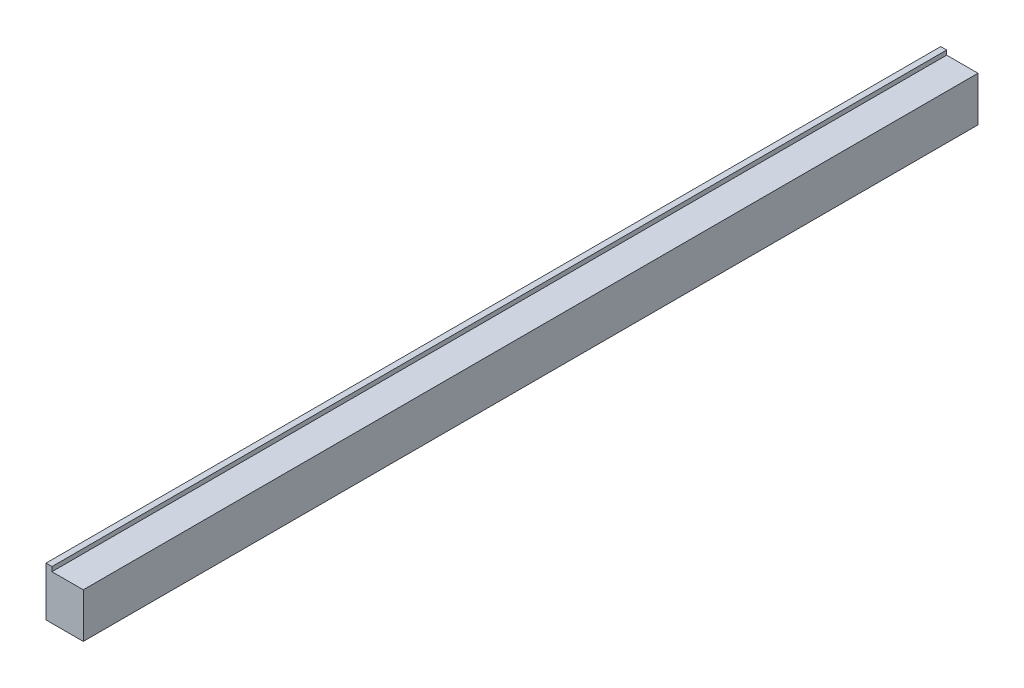
from build123d import *

# Parameters (mm, degrees)
EXTRUDE_1_DEPTH = 600


with BuildPart() as part:
    # 草图1 → 凸台-拉伸1 (new body)
    with BuildSketch(Plane.XY.offset(-300)):
        Polygon((-10, -12.5), (-14, -12.5), (-14, -45.5), (11, -45.5), (11, -15.5), (-10, -15.5), align=None)
    extrude(amount=-EXTRUDE_1_DEPTH)


solid = part.part
